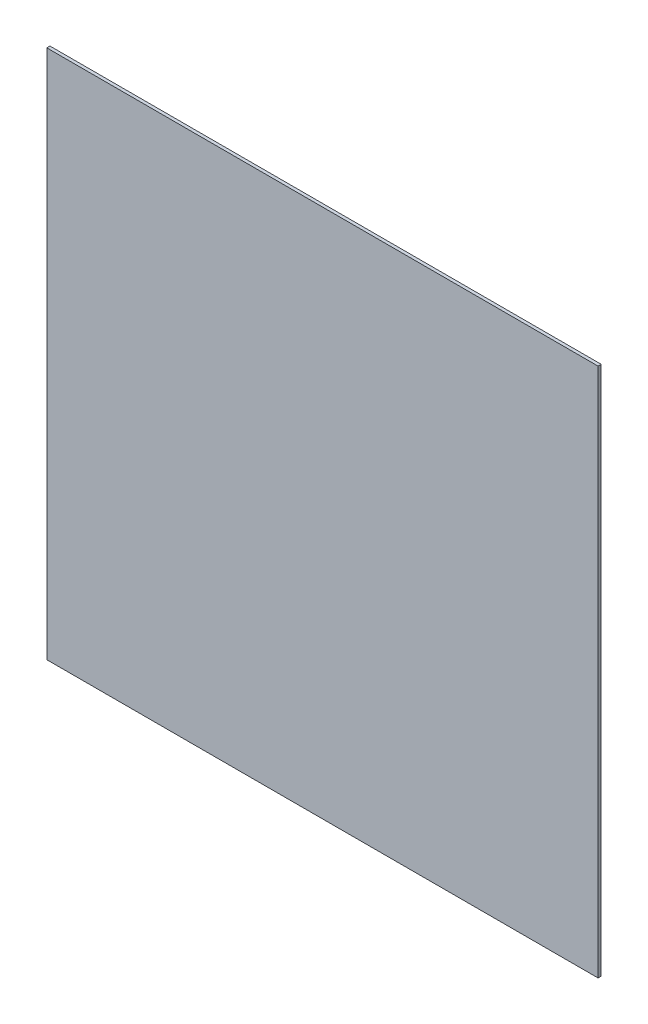
from build123d import *

# Parameters (mm, degrees)
SKETCH_1_W      = 876
SKETCH_1_H      = 842
EXTRUDE_1_DEPTH = 5


with BuildPart() as part:
    # 草图1 → 凸台-拉伸1 (new body)
    with BuildSketch(Plane.XY):
        Rectangle(SKETCH_1_W, SKETCH_1_H)
    extrude(amount=EXTRUDE_1_DEPTH)


solid = part.part
